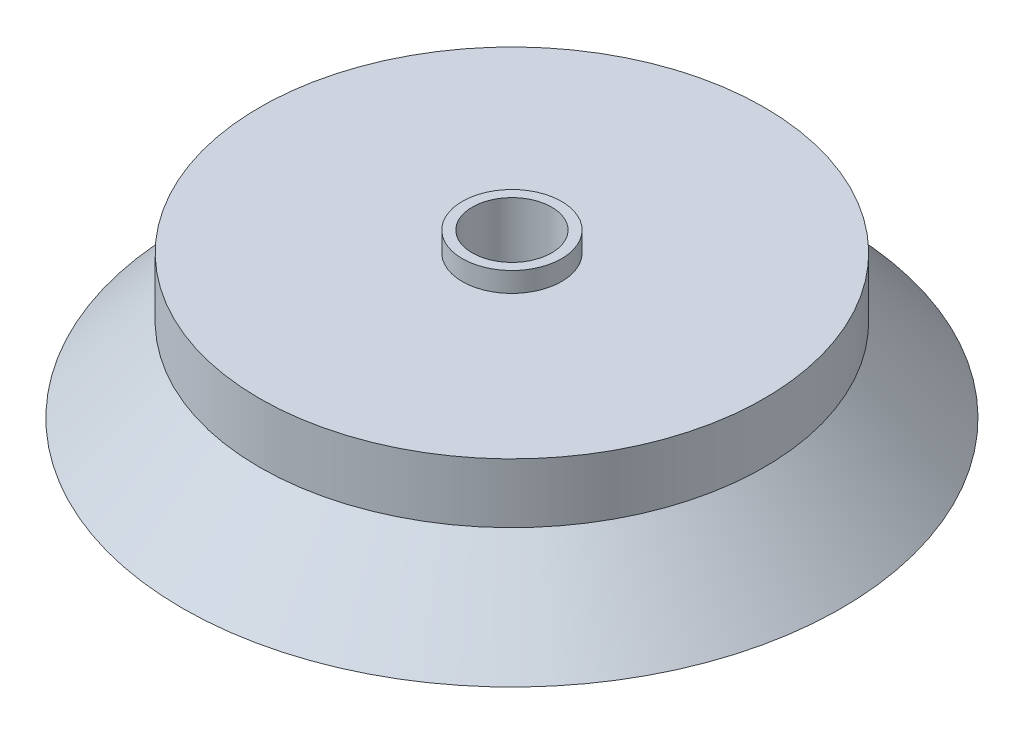
from build123d import *


with BuildPart() as part:
    # 草图1 → 旋转1 (revolve)
    with BuildSketch(Plane.XY, mode=Mode.PRIVATE) as revolve_1_sk:
        Polygon((-6.25, 17.813596491), (-5, 17.813596491), (-5, 4.34498949), (-31.981467322, 4.34498949), (-38.5, -2.686403509), (-41.5, -2.686403509), (-31.765855836, 7.813596491), (-31.765855836, 15.313596491), (-6.25, 15.313596491), align=None)
    revolve(revolve_1_sk.sketch.rotate(Axis((0, 20.559210526, 0), (0, -1, 0)), 270), axis=Axis((0, 20.559210526, 0), (0, -1, 0)))


solid = part.part
